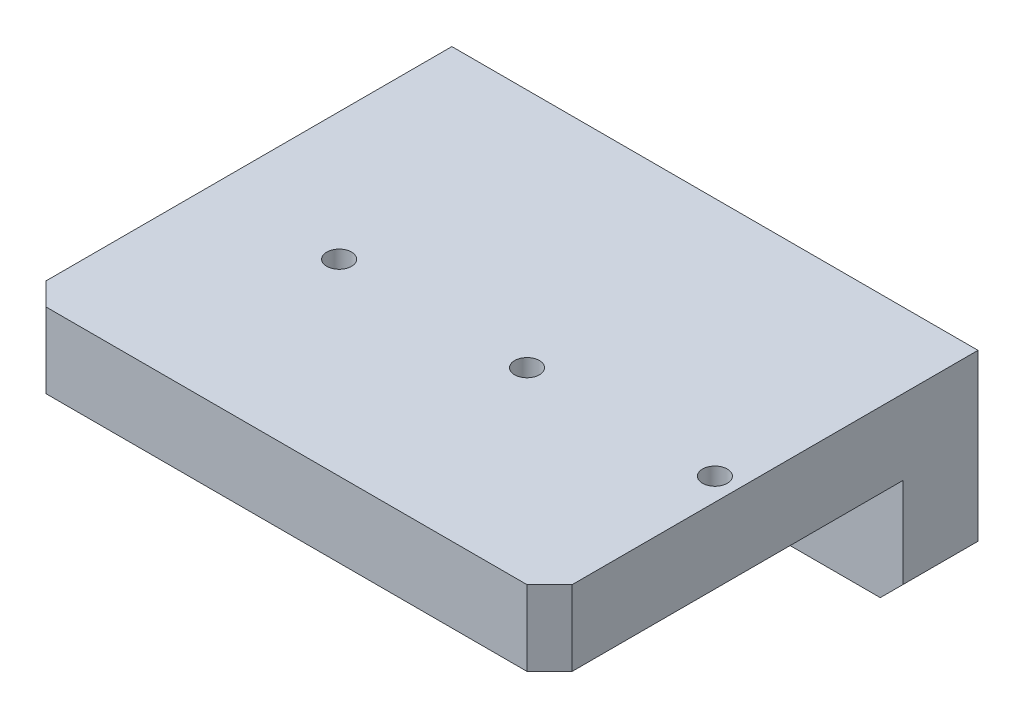
SolidWorks part; units mm, degrees
material "A6061 T6"
ref_plane "前视基准面" through (0, 0, 0) normal (0, 0, 1) x (1, 0, 0)
ref_plane "上视基准面" through (0, 0, 0) normal (0, 1, 0) x (1, 0, 0)
ref_plane "右视基准面" through (0, 0, 0) normal (1, 0, 0) x (0, 0, -1)
sketch "草图1" plane through (0, 0, 0) normal (0, 1, 0) x (1, 0, 0)
  line L1 (-35, 28.5) -> (35, 28.5)
  line L2 (-35, 28.5) -> (-35, -28.5)
  line L3 (-35, -28.5) -> (35, -28.5)
  line L4 (35, 28.5) -> (35, -28.5)
  line L5 (-35, 28.5) -> (35, -28.5) construction
  line L6 (-35, -28.5) -> (35, 28.5) construction
  point P0 (0, 0)
  dimension "D1" = 70
  dimension "D2" = 57
extrude "凸台-拉伸1" add sketch "草图1" along normal blind 10
sketch "草图2" plane through (0, 0, 0) normal (0, -1, 0) x (1, 0, 0)
  line L0 (-35, -28.5) -> (-35, 28.5) construction
  line L1 (35, -28.5) -> (-35, -28.5)
  line L2 (35, -28.5) -> (35, -18.5)
  line L3 (35, -18.5) -> (-35, -18.5)
  line L4 (-35, -28.5) -> (-35, -18.5)
  dimension "D1" = 10
extrude "凸台-拉伸2" add sketch "草图2" along normal blind 15
chamfer "倒角1" distance 3 angle 45 4 edges at (-35, -15, -23.5) (-35, 5, 28.5) (35, 5, 28.5) (35, -15, -23.5)
hole_wizard "M4 螺纹孔1" positions "草图3" profile "草图4" tap size "M4" standard "GB"
sketch "草图3" plane through (0, 10, 0) normal (0, 1, 0) x (1, 0, 0)
  point P0 (32, -3.5)
  point P3 (-18, -3.5)
  point P6 (7, -3.5)
sketch "草图4" plane through (32, 10, 3.5) normal (1, 0, 0) x (0, 0, 1)
  line L0 (0, 0) -> (0, 11.0914)
  line L1 (0, 11.0914) -> (1.65, 10.1)
  line L2 (1.65, 10.1) -> (1.65, 0)
  line L5 (1.65, 0) -> (0, 0)
  line L10 (0, 11.0914) -> (-1.65, 10.1) construction
  line L11 (0, -6.35) -> (0, 107.95) construction
  dimension "螺纹孔钻头直径" = 3.3
  dimension "螺纹孔钻头深度" = 10.1
  dimension "导头角度" = 118
cosmetic thread "孔螺蚊线1" parameters "D1"=8, "D2"=4
cosmetic thread "孔螺蚊线2" parameters "D1"=8, "D2"=4
cosmetic thread "孔螺蚊线3" parameters "D1"=8, "D2"=4
hole_wizard "Ø5.5 (5.5) 直径孔1" positions "草图5" profile "草图6" hole size "Ø5.5" standard "GB"
sketch "草图5" plane through (0, 0, -18.5) normal (0, 0, 1) x (1, 0, 0)
  line L0 (32, -15) -> (-32, -15) construction
  line L1 (35, -12) -> (35, 0) construction
  point P0 (-15, -7.5)
  point P2 (-30, -7.5)
  dimension "D1" = 7.5
  dimension "D2" = 15
  dimension "D3" = 50
sketch "草图6" plane through (-15, -7.5, -18.5) normal (1, 0, 0) x (0, -1, 0)
  line L0 (0, 0) -> (0, 11.7524)
  line L1 (0, 11.7524) -> (2.75, 10.1)
  line L2 (2.75, 10.1) -> (2.75, 0)
  line L5 (2.75, 0) -> (0, 0)
  line L10 (0, 11.7524) -> (-2.75, 10.1) construction
  line L11 (0, -6.35) -> (0, 107.95) construction
  dimension "孔直径" = 5.5
  dimension "孔深度" = 10.1
  dimension "导头角度" = 118
